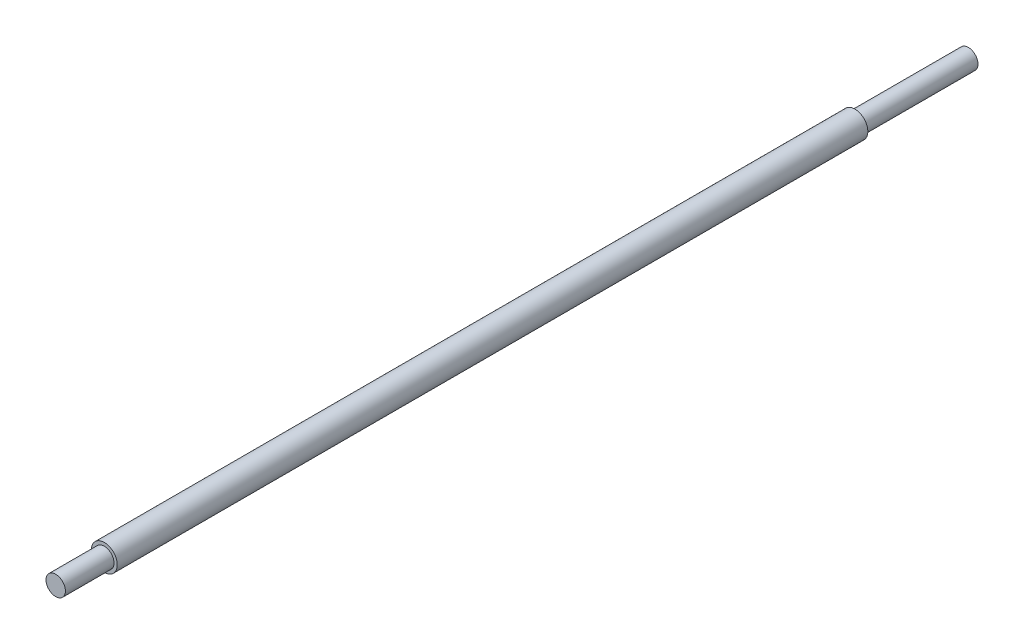
SolidWorks part; units mm, degrees
ref_plane "Front Plane" through (0, 0, 0) normal (0, 0, 1) x (1, 0, 0)
ref_plane "Top Plane" through (0, 0, 0) normal (0, 1, 0) x (1, 0, 0)
ref_plane "Right Plane" through (0, 0, 0) normal (1, 0, 0) x (0, 0, -1)
sketch "Sketch1" plane through (0, 0, 0) normal (0, 0, 1) x (1, 0, 0)
  circle A0 centre (0, 0) radius 8
  dimension "D1" = 16
extrude "Boss-Extrude1" add sketch "Sketch1" along normal mid plane 463.4
sketch "Sketch2" plane through (0, 0, 231.7) normal (0, 0, 1) x (1, 0, 0)
  circle A0 centre (0, 0) radius 6
  dimension "D1" = 12
extrude "Boss-Extrude2" add sketch "Sketch2" along normal blind 30
sketch "Sketch4" plane through (0, 0, -231.7) normal (0, 0, -1) x (-1, 0, 0)
  circle A0 centre (0, 0) radius 6
  dimension "D1" = 12
extrude "Boss-Extrude3" add sketch "Sketch4" along normal blind 70
